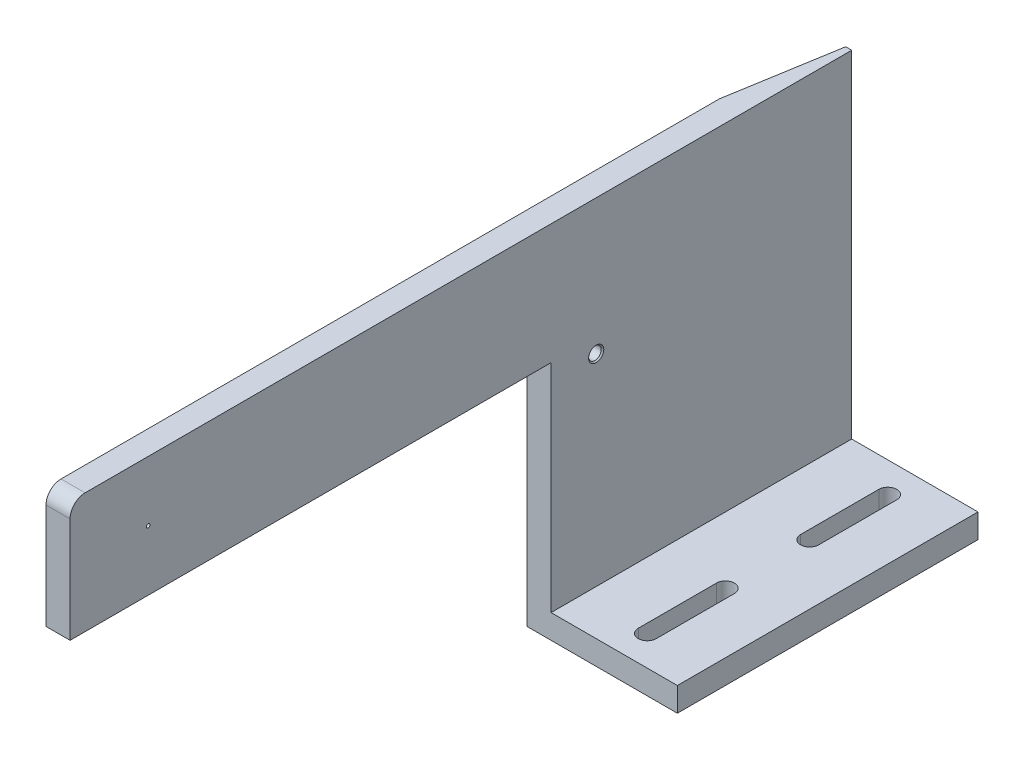
from build123d import *

# Parameters (mm, degrees)
BOSS_EXTRUDE1_DEPTH         = 260
SKETCH2_W                   = 160
SKETCH2_H                   = 80
CUT_EXTRUDE1_DEPTH          = 291.688837075
CUT_EXTRUDE2_DEPTH          = 220
CUT_EXTRUDE3_DEPTH          = 291.688837075
M5_TAPPED_HOLE1_D           = 4.2
M5_TAPPED_HOLE1_DEPTH       = 6
M5_TAPPED_HOLE1_CSINK_D     = 5.05
M5_TAPPED_HOLE1_CSINK_ANGLE = 90
M5_TAPPED_HOLE1_TIP         = 1.2618073
FILLET1_R                   = 5
SKETCH6_R                   = 0.6
CUT_EXTRUDE4_DEPTH          = 290.420109875


with BuildPart() as part:
    # Sketch1 → Boss-Extrude1 (new body)
    with BuildSketch(Plane.XY):
        Polygon((0, 0), (0, 120), (8, 120), (8, 8), (50, 8), (50, 0), align=None)
    extrude(amount=BOSS_EXTRUDE1_DEPTH)

    # Sketch2 → Cut-Extrude1 (cut, through all)
    with BuildSketch(Plane(origin=(50, 0, 0), x_dir=(0, 0, -1), z_dir=(1, 0, 0))):
        with Locations((-180, 40)):
            Rectangle(SKETCH2_W, SKETCH2_H)
    extrude(amount=-CUT_EXTRUDE1_DEPTH, mode=Mode.SUBTRACT)

    # Sketch3 → Cut-Extrude2 (cut)
    with BuildSketch(Plane(origin=(0, 8, 0), x_dir=(1, 0, 0), z_dir=(0, 1, 0))):
        with BuildLine():
            Line((27, -90), (27, -64))
            ThreePointArc((27, -64), (30, -61), (33, -64))
            Line((33, -64), (33, -90))
            ThreePointArc((33, -90), (30, -93), (27, -90))
        make_face()
        with BuildLine():
            Line((27, -36), (27, -10))
            ThreePointArc((27, -10), (30, -7), (33, -10))
            Line((33, -10), (33, -36))
            ThreePointArc((33, -36), (30, -39), (27, -36))
        make_face()
    extrude(amount=-CUT_EXTRUDE2_DEPTH, mode=Mode.SUBTRACT)

    # Sketch4 → Cut-Extrude3 (cut, through all)
    with BuildSketch(Plane(origin=(0, 120, 0), x_dir=(1, 0, 0), z_dir=(0, 1, 0))):
        Polygon((6, 0), (0, -36), (0, 0), align=None)
    extrude(amount=-CUT_EXTRUDE3_DEPTH, mode=Mode.SUBTRACT)

    # M5 Tapped Hole1
    with Locations(Plane(origin=(8, 75, 85), x_dir=(0, 0, 1), z_dir=(1, 0, 0))):
        with Locations((0, 0)):
            CounterSinkHole(M5_TAPPED_HOLE1_D / 2, M5_TAPPED_HOLE1_CSINK_D / 2, depth=M5_TAPPED_HOLE1_DEPTH, counter_sink_angle=M5_TAPPED_HOLE1_CSINK_ANGLE)
            with Locations((0, 0, -(M5_TAPPED_HOLE1_DEPTH + M5_TAPPED_HOLE1_TIP / 2))):  # 118° drill point
                Cone(0, M5_TAPPED_HOLE1_D / 2, M5_TAPPED_HOLE1_TIP, mode=Mode.SUBTRACT)

    # Fillet1
    fillet1_edges = [part.edges().sort_by_distance(p)[0] for p in [
        (4, 120, 260),
    ]]
    fillet(fillet1_edges, radius=FILLET1_R)

    # Sketch6 → Cut-Extrude4 (cut, through all)
    with BuildSketch(Plane(origin=(8, 0, 0), x_dir=(0, 0, -1), z_dir=(1, 0, 0))):
        with Locations((-234, 100)):
            Circle(SKETCH6_R)
    extrude(amount=-CUT_EXTRUDE4_DEPTH, mode=Mode.SUBTRACT)


solid = part.part
